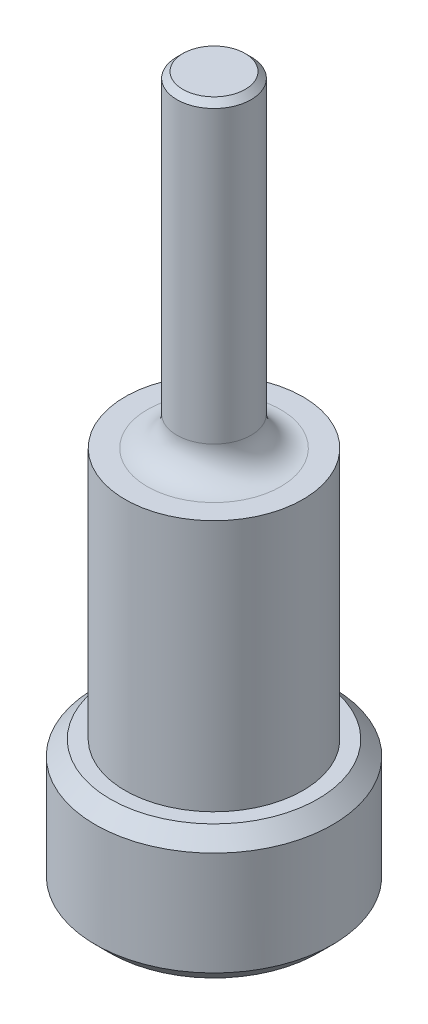
SolidWorks part; units mm, degrees
material "AL6061"
ref_plane "前视基准面" through (0, 0, 0) normal (0, 0, 1) x (1, 0, 0)
ref_plane "上视基准面" through (0, 0, 0) normal (0, 1, 0) x (1, 0, 0)
ref_plane "右视基准面" through (0, 0, 0) normal (1, 0, 0) x (0, 0, -1)
sketch "草图1" plane through (0, 0, 0) normal (0, 0, 1) x (1, 0, 0)
  line L0 (0, -0.5244) -> (0, 31.2009) construction
  line L1 (1.25, 24) -> (1.25, 13)
  line L2 (0, 0) -> (4, 0)
  line L3 (0, 0) -> (0, 24)
  line L4 (0, 24) -> (1.25, 24)
  line L5 (4, 0) -> (4, 4.5)
  line L6 (1.25, 13) -> (3, 13)
  line L7 (3, 13) -> (3, 4.5)
  line L8 (3, 4.5) -> (4, 4.5)
  dimension "D1" = 8
  dimension "D2" = 24
  dimension "D3" = 2.5
  dimension "D4" = 13
  dimension "D5" = 6
  dimension "D6" = 4.5
revolve "旋转1" add sketch "草图1" angle 360 about L0
chamfer "倒角1" distance 0.5 angle 45 2 edges at (0, 0, -4) (0, 4.5, -4)
fillet "圆角1" radius 1 1 edges at (0, 13, -1.25)
chamfer "倒角2" distance 0.2 angle 45 1 edges at (0, 24, -1.25)
